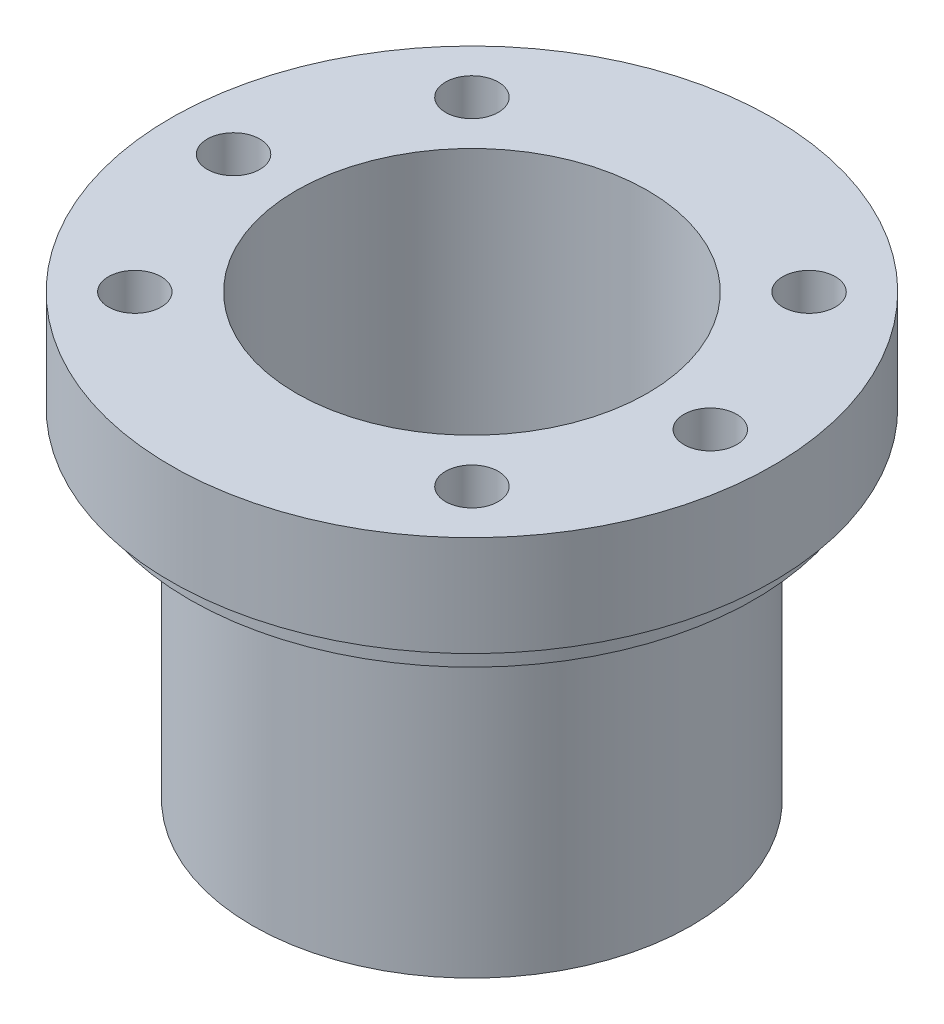
from build123d import *

# Parameters (mm, degrees)
M5_TAPPED_HOLE1_D     = 4.2
M5_TAPPED_HOLE1_DEPTH = 8.4
M5_TAPPED_HOLE1_TIP   = 1.2618073


with BuildPart() as part:
    # Sketch1 → Revolve1 (revolve)
    with BuildSketch(Plane.XY, mode=Mode.PRIVATE) as revolve1_sk:
        Polygon((14, 0), (17.5, 0), (17.5, 25), (22.5, 25), (22.5, 27), (24, 27), (24, 35), (14, 35), align=None)
    revolve(revolve1_sk.sketch.rotate(Axis((0, 0, 0), (0, 1, 0)), 90), axis=Axis((0, 0, 0), (0, 1, 0)))

    # M5 Tapped Hole1
    with Locations(Plane(origin=(0, 35, 0), x_dir=(1, 0, 0), z_dir=(0, 1, 0))):
        with Locations((-19, 0), (19, 0), (13.435028843, 13.435028843), (13.435028843, -13.435028843), (-13.435028843, -13.435028843), (-13.435028843, 13.435028843)):
            Hole(M5_TAPPED_HOLE1_D / 2, depth=M5_TAPPED_HOLE1_DEPTH)
            with Locations((0, 0, -(M5_TAPPED_HOLE1_DEPTH + M5_TAPPED_HOLE1_TIP / 2))):  # 118° drill point
                Cone(0, M5_TAPPED_HOLE1_D / 2, M5_TAPPED_HOLE1_TIP, mode=Mode.SUBTRACT)


solid = part.part
